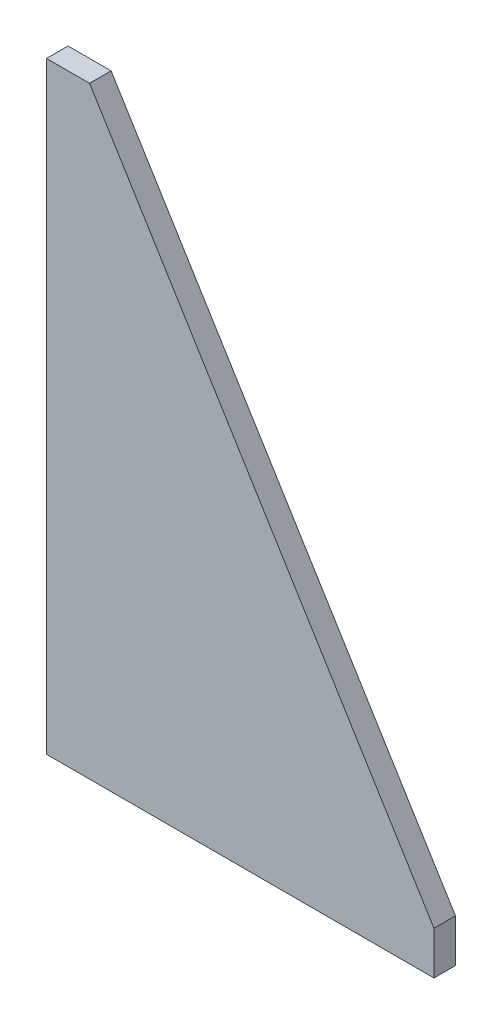
from build123d import *

# Parameters (mm, degrees)
BOSS_EXTRUDE1_DEPTH = 10


with BuildPart() as part:
    # Sketch1 → Boss-Extrude1 (new body)
    with BuildSketch(Plane.XY):
        Polygon((0, 0), (0, 280), (20, 280), (180, 20), (180, 0), align=None)
    extrude(amount=BOSS_EXTRUDE1_DEPTH)


solid = part.part
